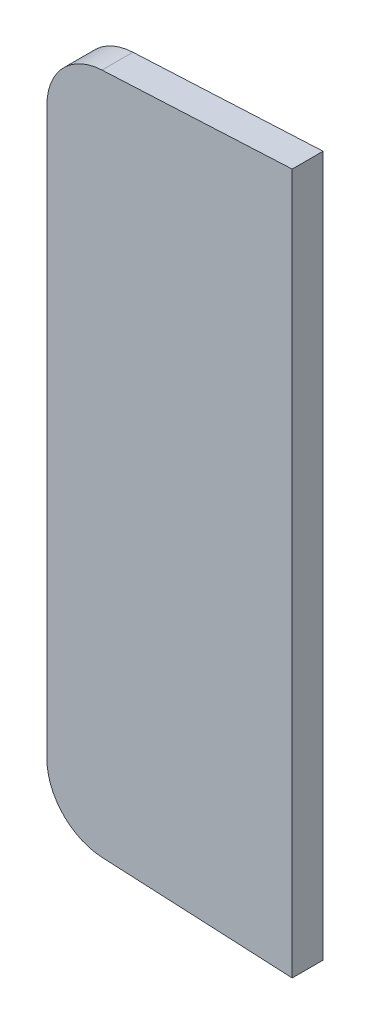
SolidWorks part; units mm, degrees
material "普通碳钢"
ref_plane "Front Plane" through (0, 0, 0) normal (0, 0, 1) x (1, 0, 0)
ref_plane "Top Plane" through (0, 0, 0) normal (0, 1, 0) x (1, 0, 0)
ref_plane "Right Plane" through (0, 0, 0) normal (1, 0, 0) x (0, 0, -1)
sketch "Sketch1" plane through (0, 0, 0) normal (0, 0, 1) x (1, 0, 0)
  line L0 (-31.75, 73.2682) -> (-31.75, -73.2682)
  line L1 (-36.4881, 0) -> (38.3494, 0) construction
  line L2 (-17.488, 88.25) -> (31.75, 90.6754)
  line L3 (-17.488, -88.25) -> (31.75, -90.6754)
  line L4 (31.75, 90.6754) -> (31.75, -90.6754)
  arc A0 (-31.75, -73.2682) -> (-17.488, -88.25) centre (-16.75, -73.2682) ccw
  arc A1 (-31.75, 73.2682) -> (-17.488, 88.25) centre (-16.75, 73.2682) cw
  point P9 (-31.75, -87.5475)
  point P12 (-31.75, 87.5475)
  dimension "D4" = 15
  dimension "D1" = 175.095
  dimension "D2" = 5.64
  dimension "D3" = 63.5
  dimension "D5" = 31.75
extrude "Boss-Extrude1" add sketch "Sketch1" along normal mid plane 8
